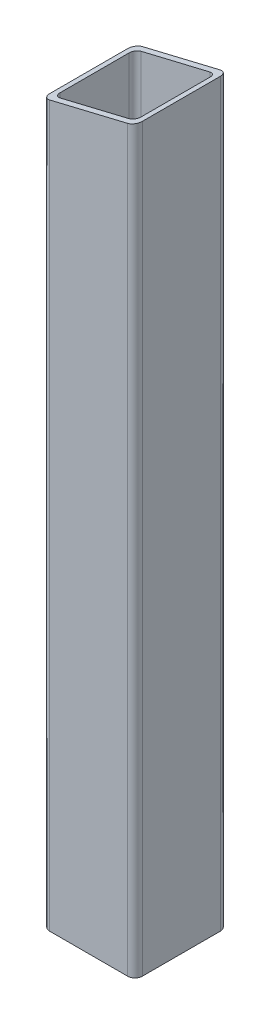
SolidWorks part; units mm, degrees
material "Angle steel 100×100×6/Q235"
ref_plane "Front Plane" through (0, 0, 0) normal (0, 0, 1) x (1, 0, 0)
ref_plane "Top Plane" through (0, 0, 0) normal (0, 1, 0) x (1, 0, 0)
ref_plane "Right Plane" through (0, 0, 0) normal (1, 0, 0) x (0, 0, -1)
sketch "Sketch2" plane through (0, 0, 0) normal (0, 1, 0) x (1, 0, 0)
  line L0 (12.6, 4.775) -> (87.4, 4.775)
  line L1 (6.3, 11.075) -> (6.3, 85.875)
  line L2 (87.4, 92.175) -> (12.6, 92.175)
  line L3 (93.7, 85.875) -> (93.7, 11.075)
  line L4 (7.875, -1.525) -> (92.125, -1.525)
  line L5 (0, 6.35) -> (0, 90.6)
  line L6 (92.125, 98.475) -> (7.875, 98.475)
  line L7 (100, 90.6) -> (100, 6.35)
  arc A0 (100, 90.6) -> (92.125, 98.475) centre (92.125, 90.6) ccw
  arc A1 (92.125, -1.525) -> (100, 6.35) centre (92.125, 6.35) ccw
  arc A2 (0, 6.35) -> (7.875, -1.525) centre (7.875, 6.35) ccw
  arc A3 (7.875, 98.475) -> (0, 90.6) centre (7.875, 90.6) ccw
  arc A4 (12.6, 92.175) -> (6.3, 85.875) centre (12.6, 85.875) ccw
  arc A5 (93.7, 85.875) -> (87.4, 92.175) centre (87.4, 85.875) ccw
  arc A6 (87.4, 4.775) -> (93.7, 11.075) centre (87.4, 11.075) ccw
  arc A7 (6.3, 11.075) -> (12.6, 4.775) centre (12.6, 11.075) ccw
extrude "Boss-Extrude1" add sketch "Sketch2" along normal mid plane 800
sketch "Sketch4" plane through (0, 0, 1.525) normal (0, 0, 1) x (1, 0, 0)
  line L0 (100, 400) -> (0, 376)
  line L1 (0, 400) -> (0, -400) construction
  line L2 (0, 376) -> (0, 400)
  line L3 (0, 400) -> (100, 400)
  dimension "D1" = 24
extrude "Cut-Extrude1" cut sketch "Sketch4" against normal up to next
